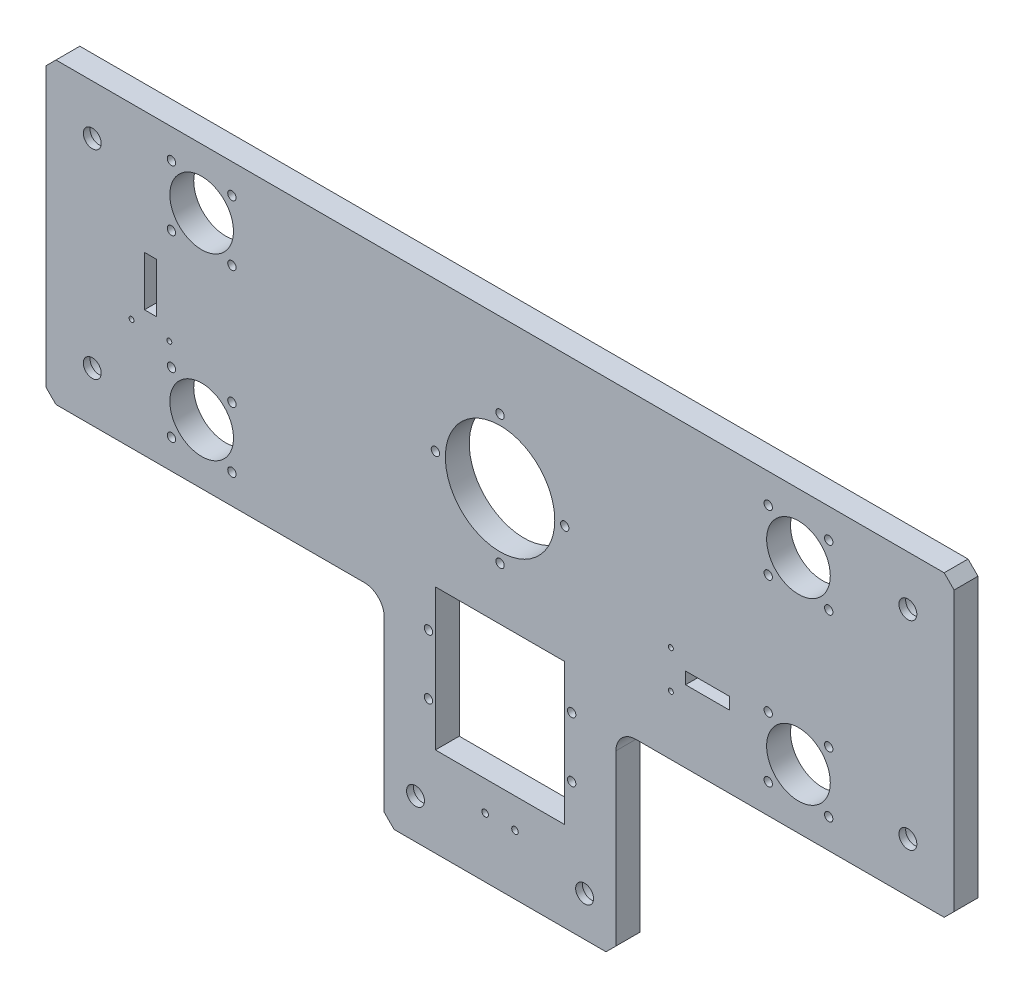
from build123d import *

# Parameters (mm, degrees)
SKETCH1_W                                           = 456.5
SKETCH1_H                                           = 250
BOSS_EXTRUDE1_DEPTH                                 = 6
SKETCH2_W                                           = 170
SKETCH2_H                                           = 100
CUT_EXTRUDE1_DEPTH                                  = 12
SKETCH3_R                                           = 16
CUT_EXTRUDE2_DEPTH                                  = 261.513075488
M5_TAPPED_HOLE1_D                                   = 4.2
SKETCH6_R                                           = 27.5
CUT_EXTRUDE3_DEPTH                                  = 261.513075488
M5_TAPPED_HOLE2_D                                   = 4.2
SKETCH9_W                                           = 65
SKETCH9_H                                           = 71
CUT_EXTRUDE4_DEPTH                                  = 261.513075488
M5_TAPPED_HOLE3_D                                   = 4.2
M4_TAPPED_HOLE1_D                                   = 3.3
SKETCH14_W                                          = 22
SKETCH14_H                                          = 6
SKETCH14_W_2                                        = 6
SKETCH14_H_2                                        = 25
CUT_EXTRUDE5_DEPTH                                  = 261.513075488
M3_TAPPED_HOLE1_D                                   = 2.5
FILLET1_R                                           = 10
CHAMFER1_SIZE                                       = 5
CBORE_FOR_M8_HEX_SOCKET_HEAD_CAP_SCREW1_D           = 9
CBORE_FOR_M8_HEX_SOCKET_HEAD_CAP_SCREW1_CBORE_D     = 15
CBORE_FOR_M8_HEX_SOCKET_HEAD_CAP_SCREW1_CBORE_DEPTH = 8.6


with BuildPart() as part:
    # Sketch1 → Boss-Extrude1 (new, symmetric)
    with BuildSketch(Plane.XY):
        Rectangle(SKETCH1_W, SKETCH1_H)
    extrude(amount=BOSS_EXTRUDE1_DEPTH, both=True)

    # Sketch2 → Cut-Extrude1 (cut)
    with BuildSketch(Plane.XY.offset(6)):
        with Locations((-143.25, -75)):
            Rectangle(SKETCH2_W, SKETCH2_H)
        with Locations((143.25, -75)):
            Rectangle(SKETCH2_W, SKETCH2_H)
    extrude(amount=-CUT_EXTRUDE1_DEPTH, mode=Mode.SUBTRACT)

    # Sketch3 → Cut-Extrude2 (cut, through all)
    with BuildSketch(Plane.XY.offset(6)):
        with Locations((150, 95)):
            Circle(SKETCH3_R)
        with Locations((150, 5)):
            Circle(SKETCH3_R)
        with Locations(Location((-150, 5, 0), (0, 0, 180))):
            Circle(SKETCH3_R)
        with Locations(Location((-150, 95, 0), (0, 0, 180))):
            Circle(SKETCH3_R)
    extrude(amount=-CUT_EXTRUDE2_DEPTH, mode=Mode.SUBTRACT)

    # M5 Tapped Hole1 (through all)
    with Locations(Plane.XY.offset(6)):
        with Locations((134.797204204, 110.202795796), (165.202795796, 110.202795796), (134.797204204, 79.797204204), (165.202795796, 79.797204204), (134.797204204, 20.202795796), (165.202795796, 20.202795796), (134.797204204, -10.202795796), (165.202795796, -10.202795796), (-134.797204204, -10.202795796), (-165.202795796, -10.202795796), (-134.797204204, 20.202795796), (-165.202795796, 20.202795796), (-134.797204204, 79.797204204), (-165.202795796, 79.797204204), (-134.797204204, 110.202795796), (-165.202795796, 110.202795796)):
            Hole(M5_TAPPED_HOLE1_D / 2)

    # Sketch6 → Cut-Extrude3 (cut, through all)
    with BuildSketch(Plane.XY.offset(6)):
        with Locations((0, 50)):
            Circle(SKETCH6_R)
    extrude(amount=-CUT_EXTRUDE3_DEPTH, mode=Mode.SUBTRACT)

    # M5 Tapped Hole2 (through all)
    with Locations(Plane.XY.offset(6)):
        with Locations((32.5, 50), (0, 82.5), (-32.5, 50), (0, 17.5)):
            Hole(M5_TAPPED_HOLE2_D / 2)

    # Sketch9 → Cut-Extrude4 (cut, through all)
    with BuildSketch(Plane.XY.offset(6)):
        with Locations((0, -44.5)):
            Rectangle(SKETCH9_W, SKETCH9_H)
    extrude(amount=-CUT_EXTRUDE4_DEPTH, mode=Mode.SUBTRACT)

    # M5 Tapped Hole3 (through all)
    with Locations(Plane.XY.offset(6)):
        with Locations((36, -29.5), (36, -59.5), (-36, -59.5), (-36, -29.5)):
            Hole(M5_TAPPED_HOLE3_D / 2)

    # M4 Tapped Hole1 (through all)
    with Locations(Plane.XY.offset(6)):
        with Locations((-7.5, -95), (7.5, -95)):
            Hole(M4_TAPPED_HOLE1_D / 2)

    # Sketch14 → Cut-Extrude5 (cut, through all)
    with BuildSketch(Plane(origin=(0, 0, -6), x_dir=(-1, 0, 0), z_dir=(0, 0, -1))):
        with Locations((-104.25, 14.25)):
            Rectangle(SKETCH14_W, SKETCH14_H)
        with Locations((175.75, 51)):
            Rectangle(SKETCH14_W_2, SKETCH14_H_2)
    extrude(amount=-CUT_EXTRUDE5_DEPTH, mode=Mode.SUBTRACT)

    # M3 Tapped Hole1 (through all)
    with Locations(Plane(origin=(0, 0, -6), x_dir=(-1, 0, 0), z_dir=(0, 0, -1))):
        with Locations((-85.85, 23.75), (185.25, 31.1), (-85.85, 4.75), (166.25, 31.1)):
            Hole(M3_TAPPED_HOLE1_D / 2)

    # Fillet1
    fillet1_edges = [part.edges().sort_by_distance(p)[0] for p in [
        (-58.25, -25, 0),
        (58.25, -25, 0),
    ]]
    fillet(fillet1_edges, radius=FILLET1_R)

    # Chamfer1
    chamfer1_edges = [part.edges().sort_by_distance(p)[0] for p in [
        (-228.25, -25, 0),
        (-58.25, -125, 0),
        (228.25, -25, 0),
        (58.25, -125, 0),
        (-228.25, 125, 0),
        (228.25, 125, 0),
    ]]
    chamfer(chamfer1_edges, length=CHAMFER1_SIZE)

    # CBORE for M8 Hex Socket Head Cap Screw1 (through all)
    with Locations(Plane(origin=(0, 0, -6), x_dir=(-1, 0, 0), z_dir=(0, 0, -1))):
        with Locations((-205, 100), (-205, 0), (205, 0), (205, 100), (-42.5, -105), (42.5, -105)):
            CounterBoreHole(CBORE_FOR_M8_HEX_SOCKET_HEAD_CAP_SCREW1_D / 2, CBORE_FOR_M8_HEX_SOCKET_HEAD_CAP_SCREW1_CBORE_D / 2, CBORE_FOR_M8_HEX_SOCKET_HEAD_CAP_SCREW1_CBORE_DEPTH)


solid = part.part
